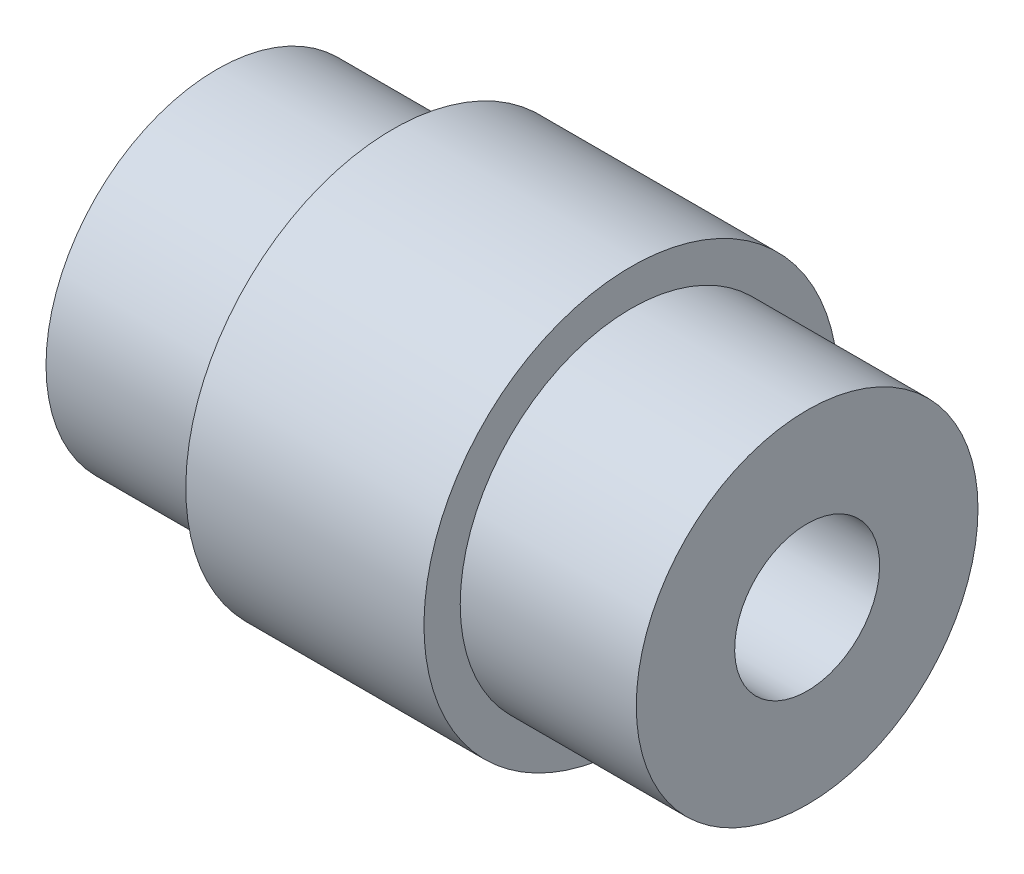
SolidWorks part; units mm, degrees
ref_plane "前视基准面" through (0, 0, 0) normal (0, 0, 1) x (1, 0, 0)
ref_plane "上视基准面" through (0, 0, 0) normal (0, 1, 0) x (1, 0, 0)
ref_plane "右视基准面" through (0, 0, 0) normal (1, 0, 0) x (0, 0, -1)
sketch "草图1" plane through (0, 0, 0) normal (0, 0, 1) x (1, 0, 0)
  line L0 (-57, -7.2919) -> (57, -7.2919)
  line L1 (-57, -7.2919) -> (-57, 25.7081)
  line L2 (-57, 25.7081) -> (-23, 25.7081)
  line L3 (-23, 25.7081) -> (-23, 32.7081)
  line L4 (-23, 32.7081) -> (23, 32.7081)
  line L5 (23, 32.7081) -> (23, 25.7081)
  line L6 (23, 25.7081) -> (57, 25.7081)
  line L7 (57, 25.7081) -> (57, -7.2919)
  line L8 (0, 9.4989) -> (0, -19.6078) construction
  dimension "D1" = 40
  dimension "D2" = 33
  dimension "D3" = 114
  dimension "D4" = 46
revolve "旋转1" add sketch "草图1" angle 360 about L0
sketch "草图2" plane through (-57, 0, 0) normal (-1, 0, 0) x (0, 0, 1)
  circle A0 centre (0, -7.2919) radius 11
  dimension "D1" = 22
extrude "切除-拉伸1" cut sketch "草图2" against normal blind 45
sketch "草图3" plane through (57, 0, 0) normal (1, 0, 0) x (0, 0, -1)
  circle A0 centre (0, -7.2919) radius 14
  dimension "D1" = 28
extrude "切除-拉伸2" cut sketch "草图3" against normal blind 45
